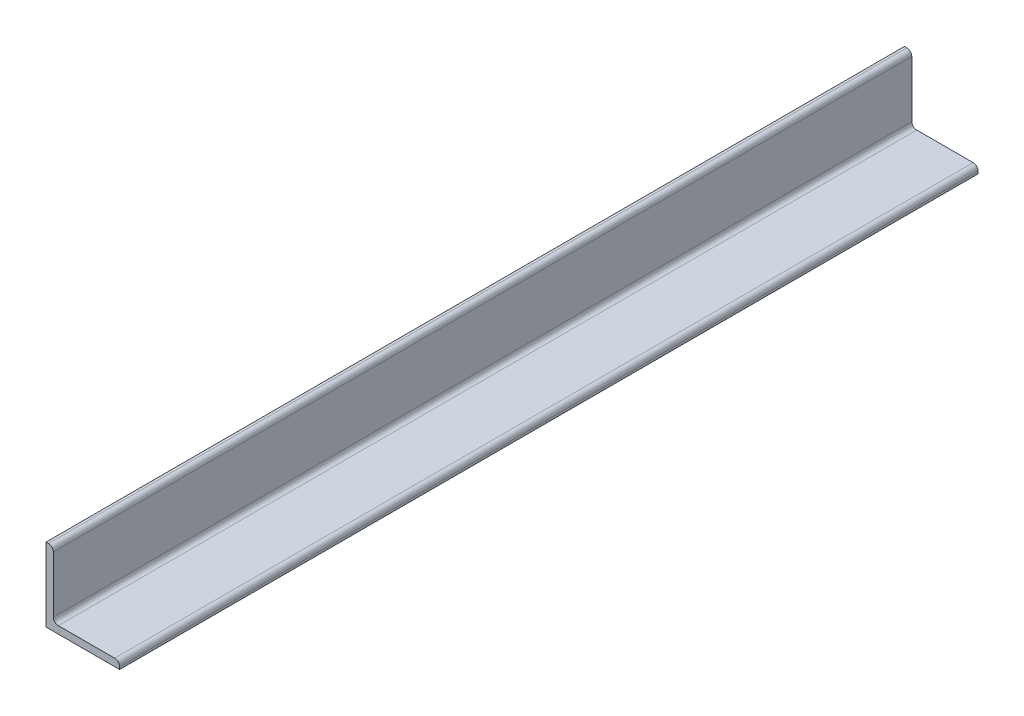
SolidWorks part; units mm, degrees
material "Plain Carbon Steel"
ref_plane "Front Plane" through (0, 0, 0) normal (0, 0, 1) x (1, 0, 0)
ref_plane "Top Plane" through (0, 0, 0) normal (0, 1, 0) x (1, 0, 0)
ref_plane "Right Plane" through (0, 0, 0) normal (1, 0, 0) x (0, 0, -1)
sketch "Sketch1" plane through (0, 0, 0) normal (0, 0, 1) x (1, 0, 0)
  line L0 (0, 0) -> (30, 0)
  line L1 (0, 0) -> (0, 30)
  line L2 (5, 3) -> (28, 3)
  line L3 (3, 5) -> (3, 28)
  line L4 (0, 30) -> (1, 30)
  line L5 (30, 1) -> (30, 0)
  line L6 (3, 3) -> (30, 3) construction
  line L7 (3, 3) -> (3, 30) construction
  arc A0 (30, 1) -> (28, 3) centre (28, 1) ccw
  arc A1 (5, 3) -> (3, 5) centre (5, 5) cw
  arc A2 (3, 28) -> (1, 30) centre (1, 28) ccw
  dimension "D4" = 2
  dimension "D1" = 30
  dimension "D2" = 30
  dimension "D3" = 3
extrude "Boss-Extrude1" add sketch "Sketch1" along normal blind 350
